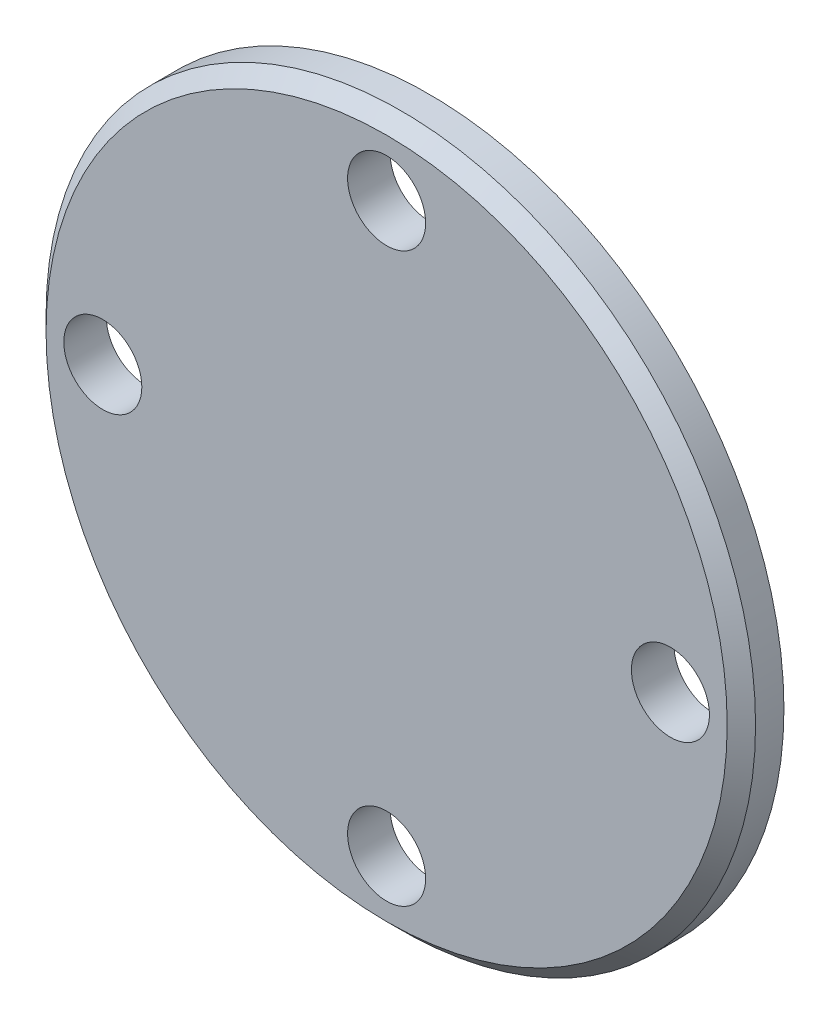
SolidWorks part; units mm, degrees
ref_plane "Front Plane" through (0, 0, 0) normal (0, 0, 1) x (1, 0, 0)
ref_plane "Top Plane" through (0, 0, 0) normal (0, 1, 0) x (1, 0, 0)
ref_plane "Right Plane" through (0, 0, 0) normal (1, 0, 0) x (0, 0, -1)
sketch "Sketch1" plane through (0, 0, 0) normal (0, 0, 1) x (1, 0, 0)
  circle A0 centre (0, 0) radius 25
  dimension "D1" = 50
extrude "Boss-Extrude1" add sketch "Sketch1" along normal blind 3
chamfer "Chamfer1" distance 1 angle 45 1 edges at (25, 0, 3)
sketch "Sketch2" plane through (0, 0, 3) normal (0, 0, 1) x (1, 0, 0)
  line L0 (0, 0) -> (20, 0) construction
  circle A0 centre (20, 0) radius 2.75
  circle A1 centre (0, -20) radius 2.75
  circle A2 centre (-20, 0) radius 2.75
  circle A3 centre (0, 20) radius 2.75
  point P12 (0, 0)
  dimension "D2" = 5.5
  dimension "D1" = 20
  dimension "D3" = 4
extrude "Cut-Extrude1" cut sketch "Sketch2" against normal blind 3
